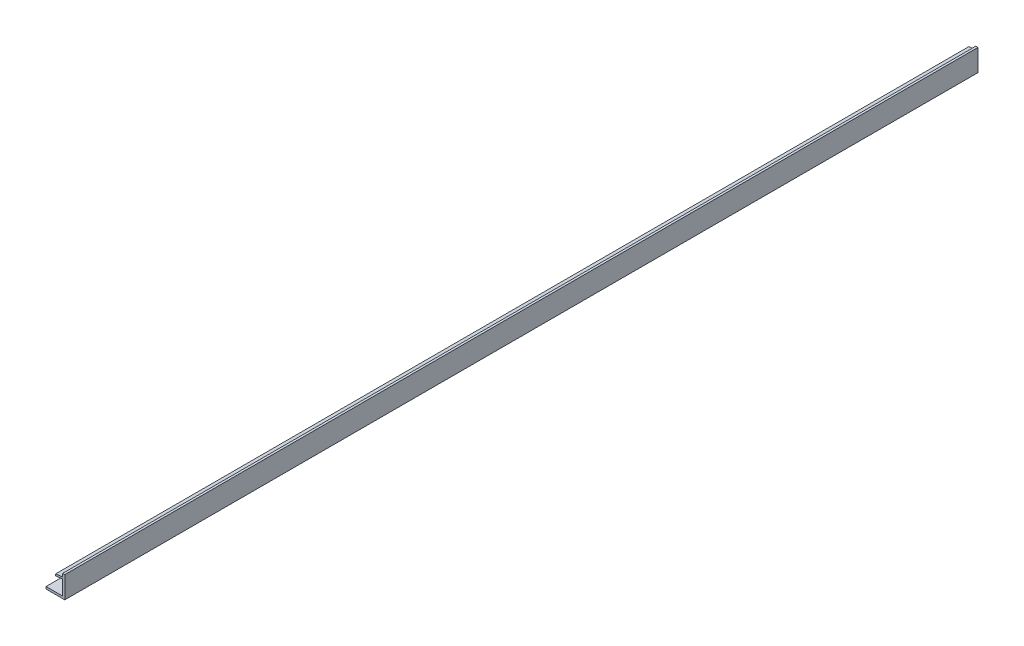
SolidWorks part; units mm, degrees
material "A3"
ref_plane "前视基准面" through (0, 0, 0) normal (0, 0, 1) x (1, 0, 0)
ref_plane "上视基准面" through (0, 0, 0) normal (0, 1, 0) x (1, 0, 0)
ref_plane "右视基准面" through (0, 0, 0) normal (1, 0, 0) x (0, 0, -1)
sketch "草图1" plane through (0, 0, 0) normal (0, 0, 1) x (1, 0, 0)
  line L0 (-43, 0) -> (0, 0)
  line L1 (0, 0) -> (0, 50)
  line L2 (-43, 5) -> (-5, 5)
  line L3 (-5, 5) -> (-5, 50)
  line L4 (-43, 5) -> (-43, 0)
  line L5 (0, 50) -> (-5, 50)
  dimension "D1" = 50
  dimension "D2" = 43
  dimension "D3" = 5
extrude "凸台-拉伸1" add sketch "草图1" along normal mid plane 2090
sketch "草图2" plane through (0, 0, 0) normal (0, 0, 1) x (1, 0, 0)
  line L0 (-5, 43.0311) -> (-21, 41.0311)
  line L1 (-5, 50) -> (-5, 5) construction
  line L2 (-21, 41.0311) -> (-21, 37)
  line L3 (-21, 37) -> (-5, 39)
  line L4 (-5, 39) -> (-5, 43.0311)
  dimension "D1" = 2
  dimension "D2" = 4
  dimension "D3" = 39
  dimension "D4" = 16
extrude "凸台-拉伸2" add sketch "草图2" along normal mid plane 2090 separate body
